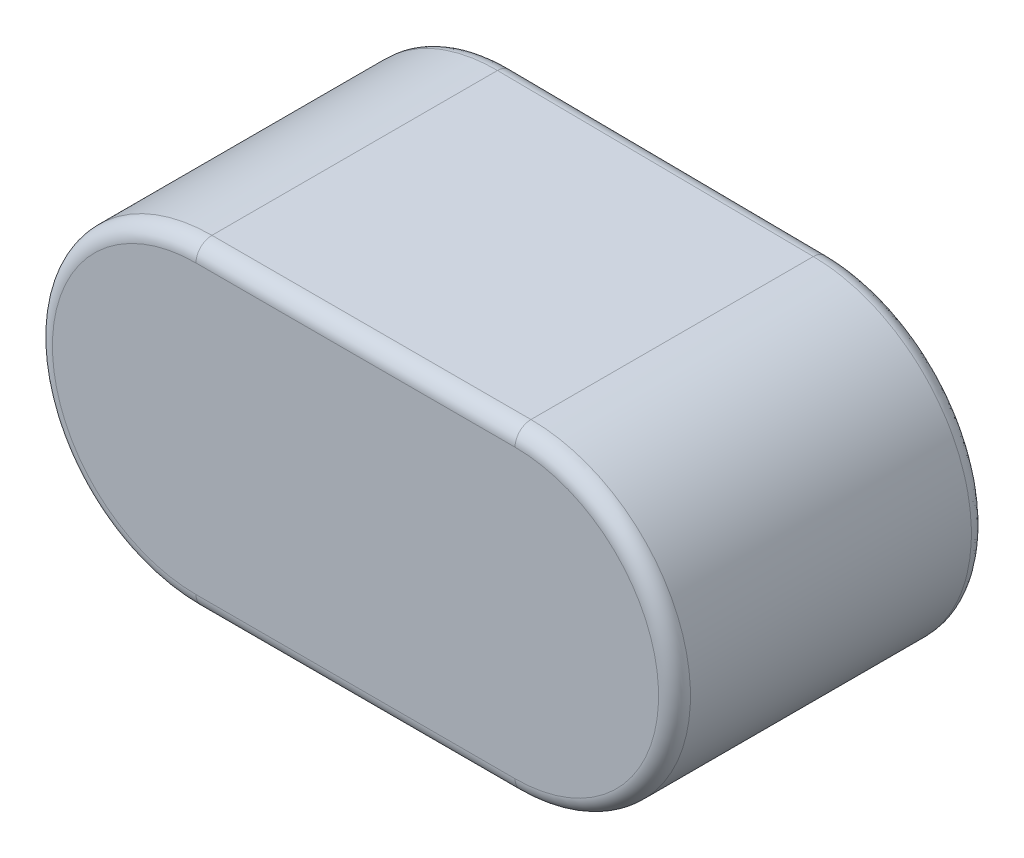
from build123d import *

# Parameters (mm, degrees)
EXTRUDE1_DEPTH          = 5
CUT_EXTRUDE1_DEPTH      = 8.5
CUT_EXTRUDE1_DEPTH_BACK = 8.5
FILLET2_R               = 0.25


with BuildPart() as part:
    # Sketch1 → Extrude1 (new body)
    with BuildSketch(Plane.XY):
        with BuildLine():
            Line((-2.5, 2.5), (2.5, 2.5))
            ThreePointArc((2.5, 2.5), (5, 0), (2.5, -2.5))
            Line((2.5, -2.5), (-2.5, -2.5))
            ThreePointArc((-2.5, -2.5), (-5, 0), (-2.5, 2.5))
        make_face()
    extrude(amount=EXTRUDE1_DEPTH)

    # Sketch2 → Cut-Extrude1 (cut, two sides: drawn at the far end of the back side and taken through both)
    with BuildSketch(Plane(origin=(0, 0, 0), x_dir=(1, 0, 0), z_dir=(0, 1, 0)).offset(-CUT_EXTRUDE1_DEPTH_BACK)):
        Polygon((-5, 0), (5, 0), (5, -0.1), align=None)
    extrude(amount=CUT_EXTRUDE1_DEPTH + CUT_EXTRUDE1_DEPTH_BACK, mode=Mode.SUBTRACT)

    # Fillet2
    fillet2_edges = [part.edges().sort_by_distance(p)[0] for p in [
        (5, 0, 5),
        (0, 2.5, 5),
        (-4.267744857, -1.767789049, 0.007322551),
        (0, -2.5, 0.05),
        (4.267744857, -1.767789049, 0.092677449),
        (0, 2.5, 0.05),
        (-5, 0, 5),
        (0, -2.5, 5),
    ]]
    fillet(fillet2_edges, radius=FILLET2_R)


solid = part.part
